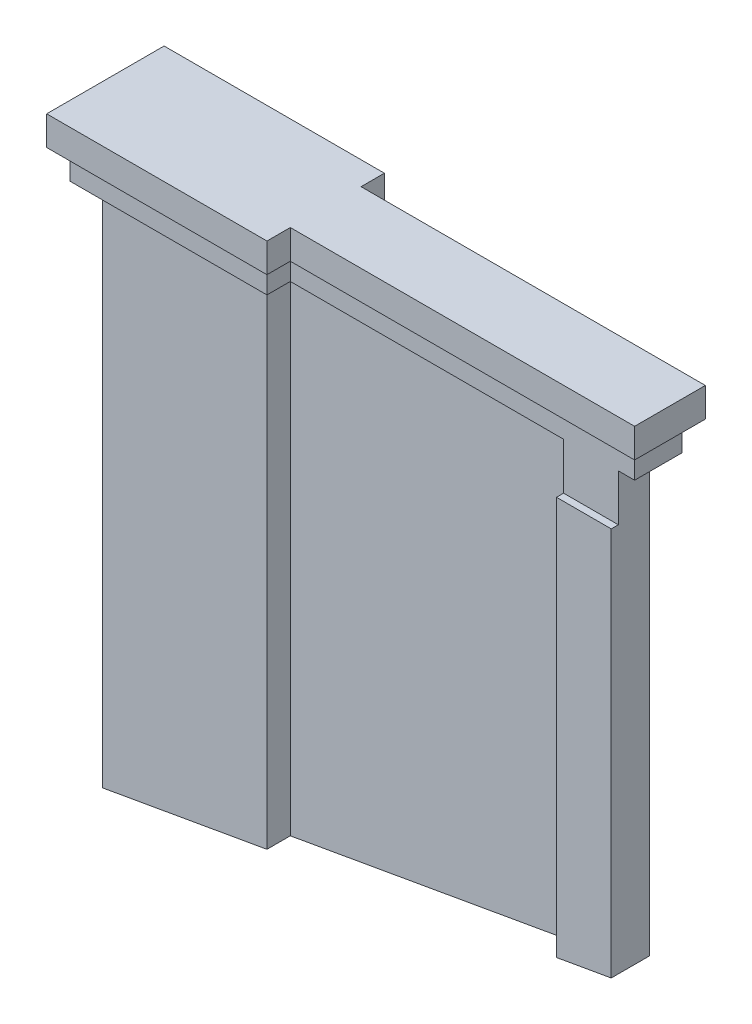
SolidWorks part; units mm, degrees
ref_plane "Front Plane" through (0, 0, 0) normal (0, 0, 1) x (1, 0, 0)
ref_plane "Top Plane" through (0, 0, 0) normal (0, 1, 0) x (1, 0, 0)
ref_plane "Right Plane" through (0, 0, 0) normal (1, 0, 0) x (0, 0, -1)
sketch "Sketch2" plane through (0, 0, 0) normal (0, 1, 0) x (1, 0, 0)
  line L0 (0, -1000) -> (0, 4.5787) construction
  line L1 (-1000, 0) -> (14.31, 0) construction
  line L2 (0.11, 0.11) -> (0.11, 5.39)
  line L3 (0.11, 5.39) -> (14.2, 5.39)
  line L4 (14.2, 5.39) -> (14.2, 3.39)
  line L5 (14.2, 3.39) -> (43.69, 3.39)
  line L6 (43.69, 3.39) -> (43.69, 0.11)
  line L7 (39, 2.11) -> (14.2, 2.11)
  line L8 (14.2, 2.11) -> (14.2, 0.11)
  line L9 (14.2, 0.11) -> (0.11, 0.11)
  line L10 (39, 0.11) -> (39, 2.11)
  line L11 (43.69, 0.11) -> (39, 0.11)
  dimension "D1" = 5.28
  dimension "D2" = 43.58
extrude "Boss-Extrude1" add sketch "Sketch2" along normal blind 45
sketch "Sketch3" plane through (0, 0, -0.11) normal (0, 0, 1) x (1, 0, 0)
  line L0 (0.11, 0) -> (43.69, 0)
  line L3 (43.69, 0) -> (43.69, 7.6843)
  line L4 (43.69, 45) -> (43.69, 0) construction
  line L5 (43.69, 7.6843) -> (0.11, 0)
  dimension "D1" = 10
extrude "Cut-Extrude1" cut sketch "Sketch3" against normal through all
sketch "Sketch4" plane through (0, 45, 0) normal (0, 1, 0) x (1, 0, 0)
  line L9 (-1.28, 6.78) -> (-1.28, -1.28)
  line L10 (-1.28, -1.28) -> (15.59, -1.28)
  line L11 (15.59, -1.28) -> (15.59, 0.72)
  line L12 (15.59, 0.72) -> (45.08, 0.72)
  line L13 (45.08, 0.72) -> (45.08, 4.78)
  line L14 (45.08, 4.78) -> (15.59, 4.78)
  line L15 (15.59, 4.78) -> (15.59, 6.78)
  line L16 (15.59, 6.78) -> (-1.28, 6.78)
extrude "Boss-Extrude2" add sketch "Sketch4" along normal blind 2.5
sketch "Sketch5" plane through (0, 47.5, 0) normal (0, 1, 0) x (1, 0, 0)
  line L5 (46.08, -0.28) -> (46.08, 5.78)
  line L8 (-2.28, 7.78) -> (-2.28, -2.28)
  line L9 (-2.28, -2.28) -> (16.59, -2.28)
  line L10 (16.59, -2.28) -> (16.59, -0.28)
  line L11 (16.59, -0.28) -> (46.08, -0.28)
  line L13 (46.08, 5.78) -> (16.59, 5.78)
  line L14 (16.59, 5.78) -> (16.59, 7.78)
  line L15 (16.59, 7.78) -> (-2.28, 7.78)
extrude "Boss-Extrude3" add sketch "Sketch5" along normal blind 2.5
sketch "Sketch6" plane through (43.69, 0, 0) normal (1, 0, 0) x (0, 0, -1)
  line L0 (0.72, 45) -> (0.72, 41)
  line L1 (0.72, 41) -> (0.11, 41)
  line L2 (0.11, 45) -> (0.11, 7.6843) construction
  line L3 (0.11, 41) -> (0.11, 45)
  line L4 (0.11, 45) -> (0.72, 45) construction
  line L5 (0.11, 45) -> (0.72, 45)
  dimension "D1" = 4
extrude "Cut-Extrude2" cut sketch "Sketch6" against normal blind 10
